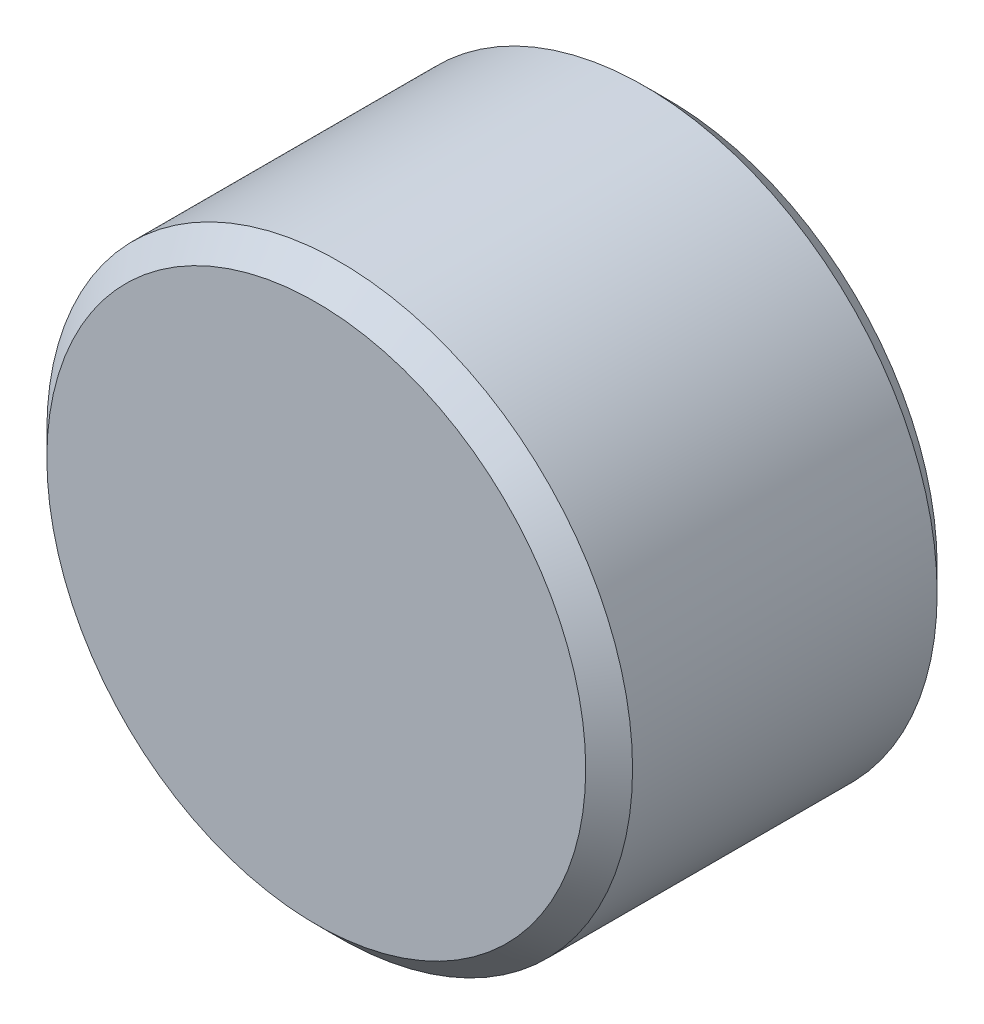
from build123d import *

# Parameters (mm, degrees)
SKETCH1_R           = 25
BOSS_EXTRUDE1_DEPTH = 30
CHAMFER1_SIZE       = 2


with BuildPart() as part:
    # Sketch1 → Boss-Extrude1 (new body)
    with BuildSketch(Plane.XY):
        Circle(SKETCH1_R)
    extrude(amount=BOSS_EXTRUDE1_DEPTH)

    # Chamfer1
    chamfer1_edges = [part.edges().sort_by_distance(p)[0] for p in [
        (-25, 0, 0),
        (-25, 0, 30),
    ]]
    chamfer(chamfer1_edges, length=CHAMFER1_SIZE)


solid = part.part
